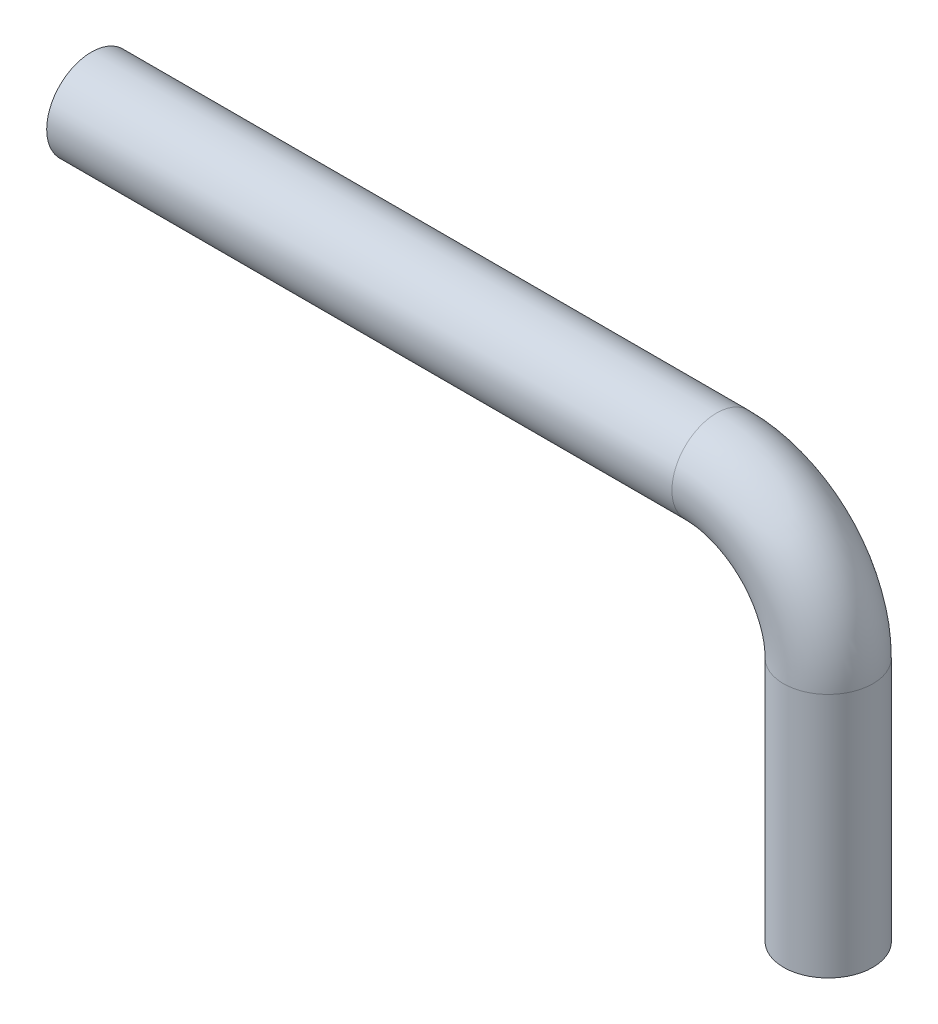
from build123d import *

# Parameters (mm, degrees)
SWEEP1_PROFILE_R = 2


with BuildPart() as part:
    # Sweep1: sweep along a path in Sketch1
    with BuildLine(Plane.XY) as sweep1_path:
        Line((0, 0), (28, 0))
        ThreePointArc((28, 0), (31.535533906, -1.464466094), (33, -5))
        Line((33, -5), (33, -16))
    # Sweep1 profile (on start of the path) → Sweep1 (sweep)
    with BuildSketch(Plane(origin=(0, 0, 0), x_dir=(0, 0, 1), z_dir=(1, 0, 0))):
        Circle(SWEEP1_PROFILE_R)
    sweep(path=sweep1_path.line)


solid = part.part
